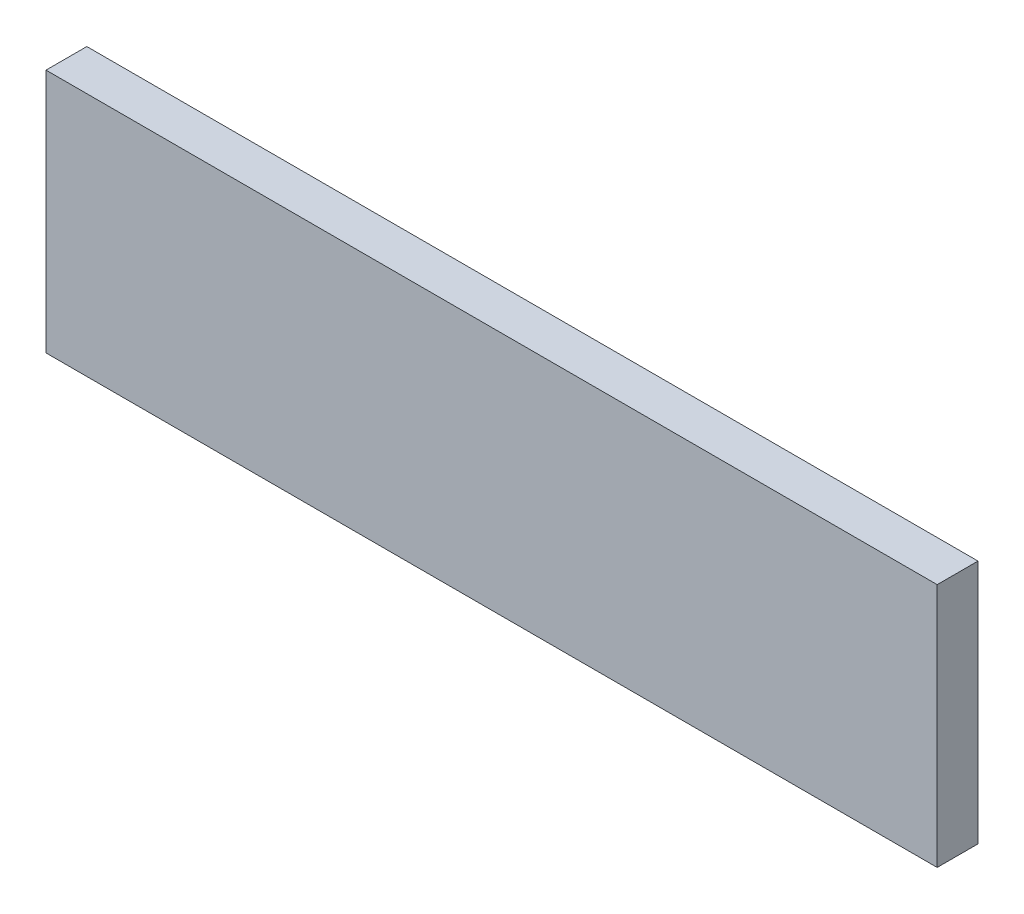
SolidWorks part; units mm, degrees
material "1023 碳钢板 (SS)"
ref_plane "前视基准面" through (0, 0, 0) normal (0, 0, 1) x (1, 0, 0)
ref_plane "上视基准面" through (0, 0, 0) normal (0, 1, 0) x (1, 0, 0)
ref_plane "右视基准面" through (0, 0, 0) normal (1, 0, 0) x (0, 0, -1)
sketch "草图1" plane through (0, 0, 0) normal (0, 0, 1) x (1, 0, 0)
  line L1 (109.15, 30) -> (-109.15, 30)
  line L2 (109.15, 30) -> (109.15, -30)
  line L3 (109.15, -30) -> (-109.15, -30)
  line L4 (-109.15, 30) -> (-109.15, -30)
  line L5 (109.15, 30) -> (-109.15, -30) construction
  line L6 (109.15, -30) -> (-109.15, 30) construction
  point P0 (0, 0)
  dimension "D1" = 218.3
  dimension "D2" = 60
extrude "凸台-拉伸1" add sketch "草图1" along normal blind 10
